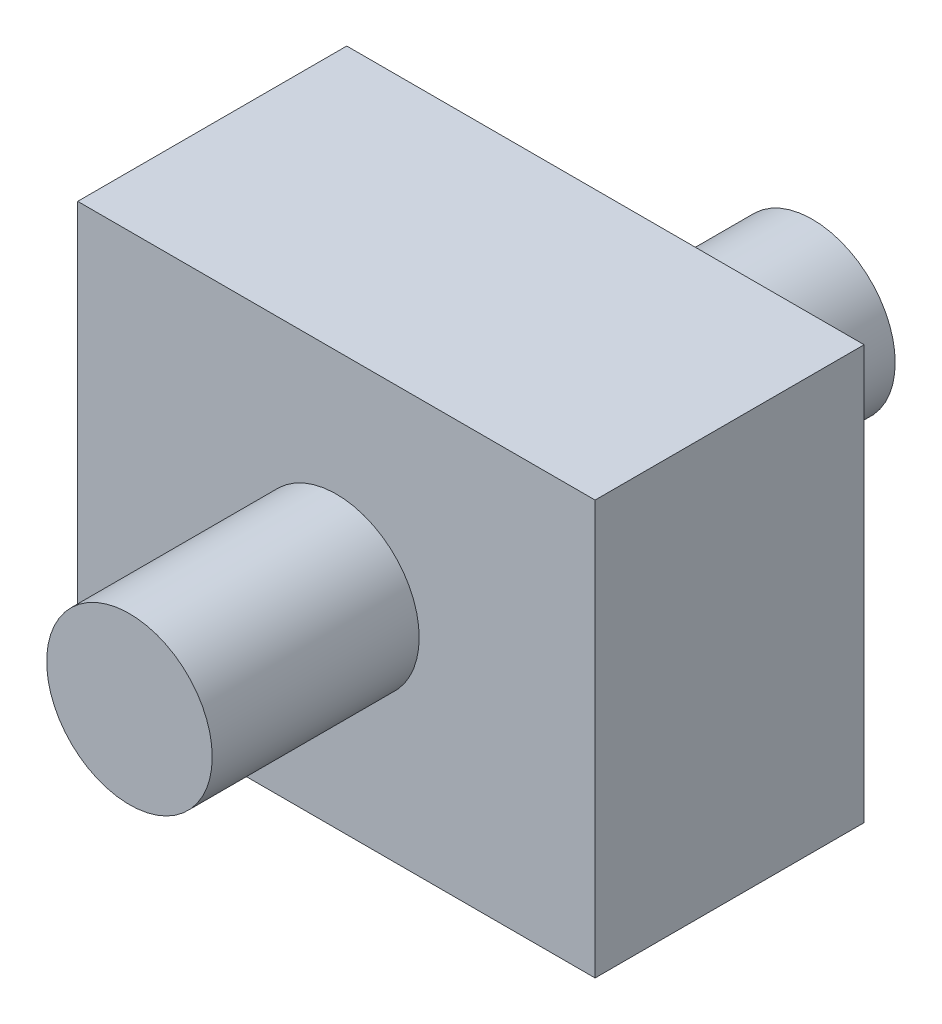
SolidWorks part; units mm, degrees
material "AISI 1045 Steel, cold drawn"
ref_plane "Front Plane" through (0, 0, 0) normal (0, 0, 1) x (1, 0, 0)
ref_plane "Top Plane" through (0, 0, 0) normal (0, 1, 0) x (1, 0, 0)
ref_plane "Right Plane" through (0, 0, 0) normal (1, 0, 0) x (0, 0, -1)
sketch "Sketch1" plane through (0, 0, 0) normal (0, 1, 0) x (1, 0, 0)
  line L1 (-12.5, -6.5) -> (12.5, -6.5)
  line L2 (-12.5, -6.5) -> (-12.5, 6.5)
  line L3 (-12.5, 6.5) -> (12.5, 6.5)
  line L4 (12.5, -6.5) -> (12.5, 6.5)
  line L5 (-12.5, -6.5) -> (12.5, 6.5) construction
  line L6 (-12.5, 6.5) -> (12.5, -6.5) construction
  point P0 (0, 0)
  dimension "D1" = 25
  dimension "D2" = 13
extrude "Boss-Extrude1" add sketch "Sketch1" along normal blind 20
sketch "Sketch2" plane through (0, 0, 6.5) normal (0, 0, 1) x (1, 0, 0)
  line L0 (12.5, 20) -> (-12.5, 0) construction
  line L1 (55, 0) -> (-55, 0) construction
  circle A0 centre (0, 10) radius 4
  dimension "D1" = 8
extrude "Boss-Extrude2" add sketch "Sketch2" along normal blind 10
mirror "Mirror1" about plane through (0, 0, 0) normal (0, 0, 1) of "Boss-Extrude2"
